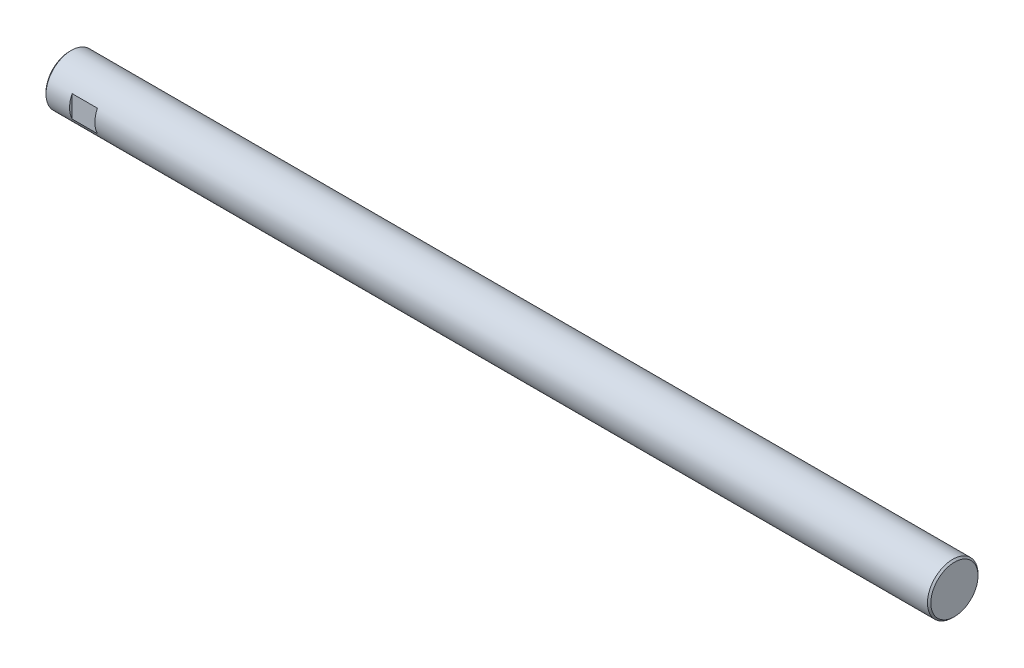
from build123d import *

# Parameters (mm, degrees)
SKETCH3_W          = 54
SKETCH3_H          = 120
SKETCH3_W_2        = 27
SKETCH3_H_2        = 60
CUT_EXTRUDE1_DEPTH = 15


with BuildPart() as part:
    # Sketch1 → Revolve1 (revolve)
    with BuildSketch(Plane.XY, mode=Mode.PRIVATE) as revolve1_sk:
        Polygon((0, 0), (0, 14), (1, 15), (524, 15), (525, 14), (525, 0), align=None)
    revolve(revolve1_sk.sketch.rotate(Axis((525, 0, 0), (-1, 0, 0)), 180), axis=Axis((525, 0, 0), (-1, 0, 0)))

    # Sketch2 → Cut-Revolve1 (revolve, cut)
    with BuildSketch(Plane.XY, mode=Mode.PRIVATE) as cut_revolve1_sk:
        Polygon((0, 0), (0, 4), (0.6765, 3.3235), (17.6, 3.3235), (19.51882362, 0), align=None)
    revolve(cut_revolve1_sk.sketch.rotate(Axis((19.51882362, 0, 0), (-1, 0, 0)), 180), axis=Axis((19.51882362, 0, 0), (-1, 0, 0)), mode=Mode.SUBTRACT)

    # Sketch3 → Cut-Extrude1 (cut)
    with BuildSketch(Plane(origin=(15, 0, 0), x_dir=(0, 0, -1), z_dir=(1, 0, 0))):
        Rectangle(SKETCH3_W, SKETCH3_H)
        Rectangle(SKETCH3_W_2, SKETCH3_H_2, mode=Mode.SUBTRACT)
    extrude(amount=CUT_EXTRUDE1_DEPTH, mode=Mode.SUBTRACT)


solid = part.part
